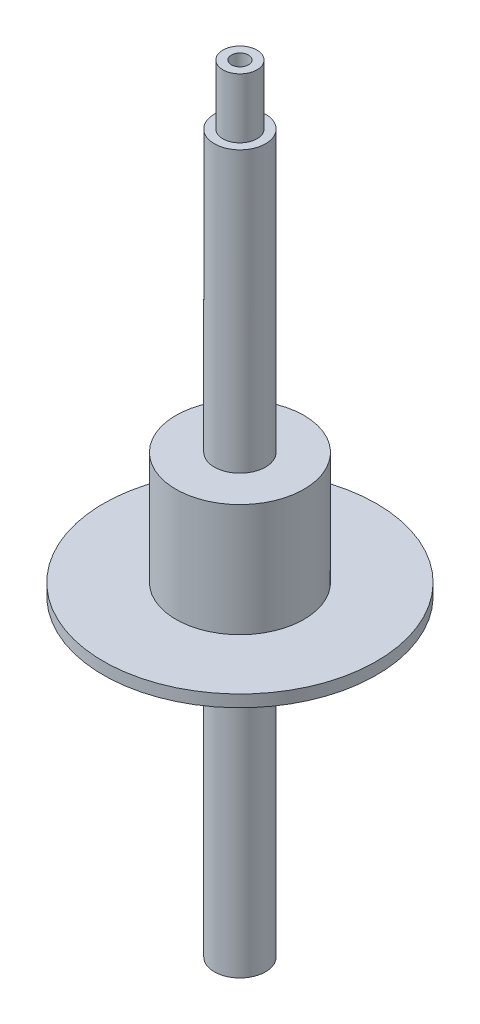
from build123d import *

# Parameters (mm, degrees)
SKETCH3_R          = 0.5
CUT_EXTRUDE1_DEPTH = 47.885498824
SKETCH4_OUTSIDE_W  = 28.164
SKETCH4_OUTSIDE_H  = 28.164
SKETCH4_OUTSIDE_R  = 1
CUT_EXTRUDE2_DEPTH = 3.5


with BuildPart() as part:
    # Sketch1 → Revolve1 (revolve)
    with BuildSketch(Plane.XY, mode=Mode.PRIVATE) as revolve1_sk:
        Polygon((0, 0), (1.5, 0), (1.5, 18.3), (8, 18.3), (8, 19), (3.75, 19), (3.75, 25.6), (1.5, 25.6), (1.5, 45.5), (0, 45.5), align=None)
    revolve(revolve1_sk.sketch.rotate(Axis((0, 0, 0), (0, 1, 0)), 90), axis=Axis((0, 0, 0), (0, 1, 0)))

    # Sketch3 → Cut-Extrude1 (cut, through all)
    with BuildSketch(Plane.XZ):
        with Locations(Location((0, 0, 0), (0, 0, 270))):
            Circle(SKETCH3_R)
    extrude(amount=-CUT_EXTRUDE1_DEPTH, mode=Mode.SUBTRACT)

    # Sketch4 outside → Cut-Extrude2 (cut)
    with BuildSketch(Plane(origin=(0, 45.5, 0), x_dir=(1, 0, 0), z_dir=(0, 1, 0))):
        Rectangle(SKETCH4_OUTSIDE_W, SKETCH4_OUTSIDE_H)
        with Locations(Location((0, 0, 0), (0, 0, 270))):
            Circle(SKETCH4_OUTSIDE_R, mode=Mode.SUBTRACT)
    extrude(amount=-CUT_EXTRUDE2_DEPTH, mode=Mode.SUBTRACT)


solid = part.part
